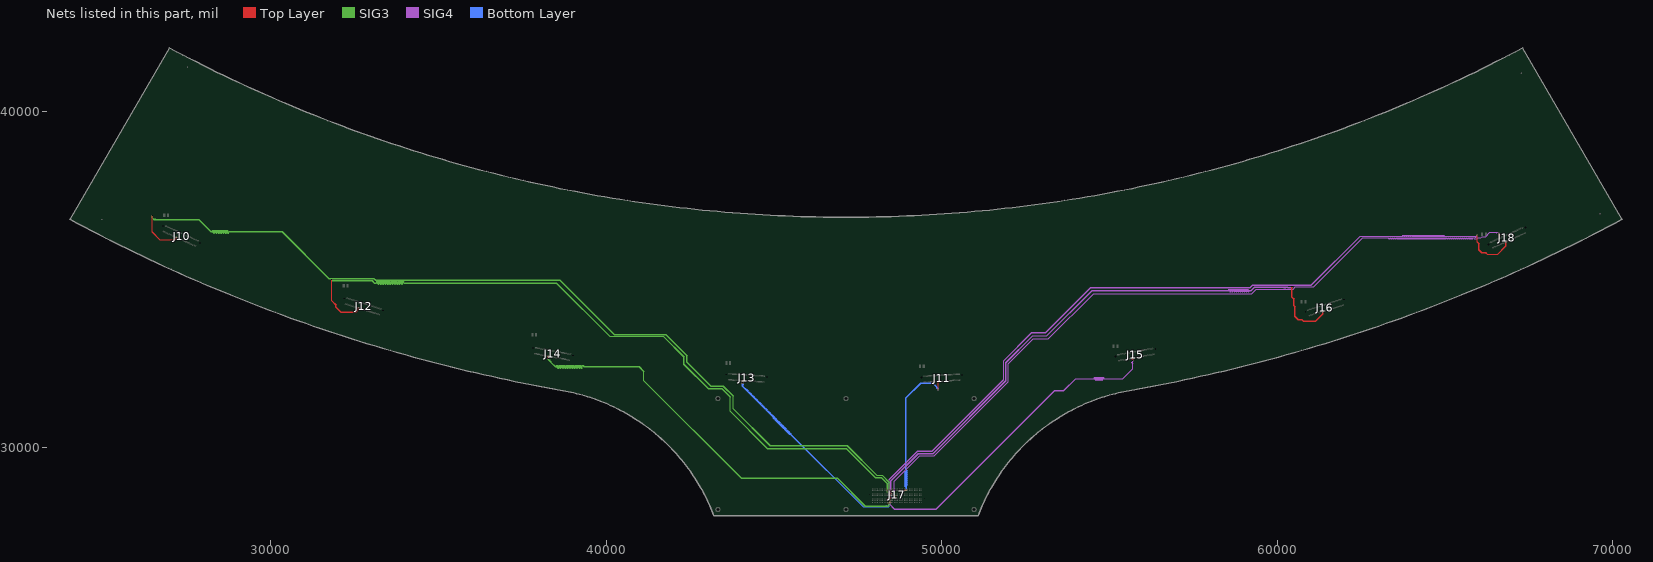
[diagram p0: the nets of this part, all layers, seen from the top]
# Altium PCB MISC86329.PcbDoc (part 7 of 11)
Units mil, origin at the board's own origin, x right, y up, seen from the top; angles counter-clockwise.
Board outline 46247.15 x 13937.21 mil, 6 copper layers (Top Layer, GND2, SIG3, SIG4, POWER5, Bottom Layer); 17 components, 210 nets, 908 pads, 1109 vias.

## Via types
v1: diameter 24, hole 12, Top Layer to Bottom Layer, 684 vias
v2: diameter 18, hole 9, Top Layer to Bottom Layer, 425 vias

## Nets (pads, with @x,y where several pads share a name; then routed paths per layer and width w, separated by ;. In a path a pad name is that pad's centre, name@x,y a point inside that pad or via, vN(x,y) a via of type N, cw(c..) or ccw(c..) an arc to the next point about the centre after c; other vN are vias at no path point) (continued)
DATAIN4P_CH7: J17.E16 J18.22 | length 23896.8
  Top Layer w5: v2(48614.09,28545) J17.E16@48637.89,28568.8 ; 66601,36381.5 66601,36360 66631.37,36329.63 J18.22@66631.37,36242.26
  SIG4 w5: v2(48614.09,28545) 48594.09,28565 48594.09,29002.09 49349,29757 49778.14,29757 51989,31967.86 51989,32495 52730,33236 53177.14,33236 54528.14,34587 59238.14,34587 59375.14,34724 60473.14,34724 60535.14,34786 61082.14,34786 62541.14,36245 63312.43,36245 63317,36240.43 63317,36225.43 63327.43,36215 63346.57,36215 63357,36225.43 63357,36240.43 63361.57,36245 63372.43,36245 63377,36240.43 63377,36225.43 63387.43,36215 63406.57,36215 63417,36225.43 63417,36240.43 63421.57,36245 63432.43,36245 63437,36240.43 63437,36225.43 63447.43,36215 63466.57,36215 63477,36225.43 63477,36240.43 63481.57,36245 63492.43,36245 63497,36240.43 63497,36225.43 63507.43,36215 63526.57,36215 63537,36225.43 63537,36240.43 63541.57,36245 63552.43,36245 63557,36240.43 63557,36225.43 63567.43,36215 63586.57,36215 63597,36225.43 63597,36240.43 63601.57,36245 63612.43,36245 63617,36240.43 63617,36225.43 63627.43,36215 63646.57,36215 63657,36225.43 63657,36240.43 63661.57,36245 63672.43,36245 63677,36240.43 63677,36225.43 63687.43,36215 63706.57,36215 63717,36225.43 63717,36240.43 63721.57,36245 63732.43,36245 63737,36240.43 63737,36225.43 63747.43,36215 63766.57,36215 63777,36225.43 63777,36240.43 63781.57,36245 63792.43,36245 63797,36240.43 63797,36225.43 63807.43,36215 63826.57,36215 63837,36225.43 63837,36240.43 63841.57,36245 63852.43,36245 63857,36240.43 63857,36225.43 63867.43,36215 63886.57,36215 63897,36225.43 63897,36240.43 63901.57,36245 63912.43,36245 63917,36240.43 63917,36225.43 63927.43,36215 63946.57,36215 63957,36225.43 63957,36240.43 63961.57,36245 63972.43,36245 63977,36240.43 63977,36225.43 63987.43,36215 64006.57,36215 64017,36225.43 64017,36240.43 64021.57,36245 64032.43,36245 64037,36240.43 64037,36225.43 64047.43,36215 64066.57,36215 64077,36225.43 64077,36240.43 64081.57,36245 64092.43,36245 64097,36240.43 64097,36225.43 64107.43,36215 64126.57,36215 64137,36225.43 64137,36240.43 64141.57,36245 64152.43,36245 64157,36240.43 64157,36225.43 64167.43,36215 64186.57,36215 64197,36225.43 64197,36240.43 64201.57,36245 64212.43,36245 64217,36240.43 64217,36225.43 64227.43,36215 64246.57,36215 64257,36225.43 64257,36240.43 64261.57,36245 64272.43,36245 64277,36240.43 64277,36225.43 64287.43,36215 64306.57,36215 64317,36225.43 64317,36240.43 64321.57,36245 64332.43,36245 64337,36240.43 64337,36225.43 64347.43,36215 64366.57,36215 64377,36225.43 64377,36240.43 64381.57,36245 64392.43,36245 64397,36240.43 64397,36225.43 64407.43,36215 64426.57,36215 64437,36225.43 64437,36240.43 64441.57,36245 64452.43,36245 64457,36240.43 64457,36225.43 64467.43,36215 64486.57,36215 64497,36225.43 64497,36240.43 64501.57,36245 64512.43,36245 64517,36240.43 64517,36225.43 64527.43,36215 64546.57,36215 64557,36225.43 64557,36240.43 64561.57,36245 64572.43,36245 64577,36240.43 64577,36225.43 64587.43,36215 64606.57,36215 64617,36225.43 64617,36240.43 64621.57,36245 64632.43,36245 64637,36240.43 64637,36225.43 64647.43,36215 64666.57,36215 64677,36225.43 64677,36240.43 64681.57,36245 64692.43,36245 64697,36240.43 64697,36225.43 64707.43,36215 64726.57,36215 64737,36225.43 64737,36240.43 64741.57,36245 64752.43,36245 64757,36240.43 64757,36225.43 64767.43,36215 64786.57,36215 64797,36225.43 64797,36240.43 64801.57,36245 64812.43,36245 64817,36240.43 64817,36225.43 64827.43,36215 64846.57,36215 64857,36225.43 64857,36240.43 64861.57,36245 64872.43,36245 64877,36240.43 64877,36225.43 64887.43,36215 64906.57,36215 64917,36225.43 64917,36240.43 64921.57,36245 64932.43,36245 64937,36240.43 64937,36225.43 64947.43,36215 64966.57,36215 64977,36225.43 64977,36240.43 64981.57,36245 64992.43,36245 64997,36240.43 64997,36225.43 65007.43,36215 65026.57,36215 65037,36225.43 65037,36240.43 65041.57,36245 65052.43,36245 65057,36240.43 65057,36225.43 65067.43,36215 65086.57,36215 65097,36225.43 65097,36240.43 65101.57,36245 65112.43,36245 65117,36240.43 65117,36225.43 65127.43,36215 65146.57,36215 65157,36225.43 65157,36240.43 65161.57,36245 65172.43,36245 65177,36240.43 65177,36225.43 65187.43,36215 65206.57,36215 65217,36225.43 65217,36240.43 65221.57,36245 65232.43,36245 65237,36240.43 65237,36225.43 65247.43,36215 65266.57,36215 65277,36225.43 65277,36240.43 65281.57,36245 65292.43,36245 65297,36240.43 65297,36225.43 65307.43,36215 65326.57,36215 65337,36225.43 65337,36240.43 65341.57,36245 65352.43,36245 65357,36240.43 65357,36225.43 65367.43,36215 65386.57,36215 65397,36225.43 65397,36240.43 65401.57,36245 65412.43,36245 65417,36240.43 65417,36225.43 65427.43,36215 65446.57,36215 65457,36225.43 65457,36240.43 65461.57,36245 65472.43,36245 65477,36240.43 65477,36225.43 65487.43,36215 65506.57,36215 65517,36225.43 65517,36240.43 65521.57,36245 65532.43,36245 65537,36240.43 65537,36225.43 65547.43,36215 65566.57,36215 65577,36225.43 65577,36240.43 65581.57,36245 65592.43,36245 65597,36240.43 65597,36225.43 65607.43,36215 65626.57,36215 65637,36225.43 65637,36240.43 65641.57,36245 65652.43,36245 65657,36240.43 65657,36225.43 65667.43,36215 65686.57,36215 65697,36225.43 65697,36240.43 65701.57,36245 65712.43,36245 65717,36240.43 65717,36225.43 65727.43,36215 65746.57,36215 65757,36225.43 65757,36240.43 65761.57,36245 65772.43,36245 65777,36240.43 65777,36225.43 65787.43,36215 65806.57,36215 65817,36225.43 65817,36240.43 65821.57,36245 65857.86,36245 65875.86,36227 65959.14,36227 65977.14,36245 66058.14,36245 66102.14,36289 66204.14,36289 66337.14,36422 66521,36422 66526,36417 66526,36402.15 66531,36397.15 66541,36397.15 66546,36402.15 66546,36417 66551,36422 66582.86,36422 66600,36404.86 66600,36396 v2@66595,36391
  other v2: 66594.5,36388
DATAIN5N_CH0: J10.29 J17.G20 | length 28227.2
  Top Layer w5: v2(26465.5,36917) 26472,36910.5 26472,36420.86 26703.86,36189 27155.14,36189 27186.72,36220.57 27186.72,36238.96 J10.29@27205.36,36257.61 ; v2(48414.09,28692.61) J17.G20@48437.89,28668.8
  SIG3 w5: v2(26465.5,36917) 26472,36910.5 26472,36846.86 26526.86,36792 26555,36792 27858.86,36792 28221.86,36429 28261.82,36429 28273.5,36440.68 28273.5,36461.49 28279.32,36467.31 28292.68,36467.31 28298.5,36461.49 28298.5,36402.37 28310.18,36390.69 28331.82,36390.69 28343.5,36402.37 28343.5,36461.49 28349.32,36467.31 28362.68,36467.31 28368.5,36461.49 28368.5,36402.37 28380.18,36390.69 28401.82,36390.69 28413.5,36402.37 28413.5,36461.49 28419.32,36467.31 28432.68,36467.31 28438.5,36461.49 28438.5,36402.37 28450.18,36390.69 28471.82,36390.69 28483.5,36402.37 28483.5,36461.49 28489.32,36467.31 28502.68,36467.31 28508.5,36461.49 28508.5,36402.37 28520.18,36390.69 28541.82,36390.69 28553.5,36402.37 28553.5,36461.49 28559.32,36467.31 28572.68,36467.31 28578.5,36461.49 28578.5,36402.37 28590.18,36390.69 28611.82,36390.69 28623.5,36402.37 28623.5,36461.49 28629.32,36467.31 28642.68,36467.31 28648.5,36461.49 28648.5,36402.37 28660.18,36390.69 28681.82,36390.69 28693.5,36402.37 28693.5,36461.49 28699.32,36467.31 28712.68,36467.31 28718.5,36461.49 28718.5,36402.37 28730.18,36390.69 28751.82,36390.69 28763.5,36402.37 28763.5,36423.18 28769.32,36429 30341.86,36429 31734.86,35036 33075.86,35036 33127.86,34984 38619.86,34984 40240.86,33363 41778,33363 42407,32734 42407,32544.86 43117.86,31834 43484,31834 43784,31534 43784,31158.86 44883.86,30059 47176,30059 48067,29168 48224.86,29168 48434.09,28958.77 48434.09,28712.61 v2(48414.09,28692.61)
DATAIN5N_CH1: J12.29 J17.F20 | length 23094.9
  Top Layer w5: v2(31815.5,35011) 31822,35004.5 31822,34375 31951,34246 31951,34175.86 32089.86,34037 32554.14,34037 32623.14,34106 32623.14,34130.56 J12.29@32643.17,34150.59 ; v2(48414.09,28642.61) J17.F20@48437.89,28618.8
  SIG3 w5: v2(31815.5,35011) 31822,35004.5 31822,34989.86 31838.86,34973 31862,34973 31867,34968 31888,34968 31893,34973 33022.86,34973 33093.86,34902 33158.82,34902 33170.5,34913.68 33170.5,34935.94 33176.32,34941.76 33189.68,34941.76 33195.5,34935.94 33195.5,34873.92 33207.18,34862.24 33228.82,34862.24 33240.5,34873.92 33240.5,34935.94 33246.32,34941.76 33259.68,34941.76 33265.5,34935.94 33265.5,34873.92 33277.18,34862.24 33298.82,34862.24 33310.5,34873.92 33310.5,34935.94 33316.32,34941.76 33329.68,34941.76 33335.5,34935.94 33335.5,34873.92 33347.18,34862.24 33368.82,34862.24 33380.5,34873.92 33380.5,34935.94 33386.32,34941.76 33399.68,34941.76 33405.5,34935.94 33405.5,34873.92 33417.18,34862.24 33438.82,34862.24 33450.5,34873.92 33450.5,34935.94 33456.32,34941.76 33469.68,34941.76 33475.5,34935.94 33475.5,34873.92 33487.18,34862.24 33508.82,34862.24 33520.5,34873.92 33520.5,34935.94 33526.32,34941.76 33539.68,34941.76 33545.5,34935.94 33545.5,34873.92 33557.18,34862.24 33578.82,34862.24 33590.5,34873.92 33590.5,34935.94 33596.32,34941.76 33609.68,34941.76 33615.5,34935.94 33615.5,34873.92 33627.18,34862.24 33648.82,34862.24 33660.5,34873.92 33660.5,34935.94 33666.32,34941.76 33679.68,34941.76 33685.5,34935.94 33685.5,34873.92 33697.18,34862.24 33718.82,34862.24 33730.5,34873.92 33730.5,34935.94 33736.32,34941.76 33749.68,34941.76 33755.5,34935.94 33755.5,34873.92 33767.18,34862.24 33788.82,34862.24 33800.5,34873.92 33800.5,34935.94 33806.32,34941.76 33819.68,34941.76 33825.5,34935.94 33825.5,34873.92 33837.18,34862.24 33858.82,34862.24 33870.5,34873.92 33870.5,34935.94 33876.32,34941.76 33889.68,34941.76 33895.5,34935.94 33895.5,34873.92 33907.18,34862.24 33928.82,34862.24 33940.5,34873.92 33940.5,34935.94 33946.32,34941.76 33959.68,34941.76 33965.5,34935.94 33965.5,34913.68 33977.18,34902 38516.86,34902 40108.86,33310 41706,33310 42318,32698 42318,32472.86 43038.86,31752 43447,31752 43694,31505 43694,31074.86 44802.86,29966 47153.86,29966 48014.86,29105 48195.86,29105 48385,28915.86 48385,28674 48406.96,28652.04 48414.09,28644.91 v2(48414.09,28642.61)
DATAIN5N_CH2: J14.29 J17.B20 | length 13805.4
  Top Layer w5: v2(38289.5,32657) 38283,32663.5 38283,32689 38293,32699 J14.29@38293,32716 ; v2(48414.09,28395) J17.B20@48437.89,28418.8
  SIG3 w5: v2@38287,32654 38282,32649 38282,32624 38296.42,32609.58 38305.26,32609.58 38308.78,32613.1 38317.62,32613.1 38326.46,32604.26 38326.46,32595.42 38322.94,32591.9 38322.94,32583.06 38331.77,32574.23 38340.61,32574.23 38344.13,32577.75 38352.97,32577.75 38361.81,32568.91 38361.81,32560.07 38358.29,32556.55 38358.29,32547.71 38490,32416 38511.68,32416 38517.5,32421.82 38517.5,32436.85 38529.18,32448.52 38550.82,32448.52 38562.5,32436.85 38562.5,32382.3 38568.32,32376.48 38581.68,32376.48 38587.5,32382.3 38587.5,32436.85 38599.18,32448.52 38620.82,32448.52 38632.5,32436.85 38632.5,32382.3 38638.32,32376.48 38651.68,32376.48 38657.5,32382.3 38657.5,32436.85 38669.18,32448.52 38690.82,32448.52 38702.5,32436.85 38702.5,32382.3 38708.32,32376.48 38721.68,32376.48 38727.5,32382.3 38727.5,32436.85 38739.18,32448.52 38760.82,32448.52 38772.5,32436.85 38772.5,32382.3 38778.32,32376.48 38791.68,32376.48 38797.5,32382.3 38797.5,32436.85 38809.18,32448.52 38830.82,32448.52 38842.5,32436.85 38842.5,32382.3 38848.32,32376.48 38861.68,32376.48 38867.5,32382.3 38867.5,32436.85 38879.18,32448.52 38900.82,32448.52 38912.5,32436.85 38912.5,32382.3 38918.32,32376.48 38931.68,32376.48 38937.5,32382.3 38937.5,32436.85 38949.18,32448.52 38970.82,32448.52 38982.5,32436.85 38982.5,32382.3 38988.32,32376.48 39001.68,32376.48 39007.5,32382.3 39007.5,32436.85 39019.18,32448.52 39040.82,32448.52 39052.5,32436.85 39052.5,32382.3 39058.32,32376.48 39071.68,32376.48 39077.5,32382.3 39077.5,32436.85 39089.18,32448.52 39110.82,32448.52 39122.5,32436.85 39122.5,32382.3 39128.32,32376.48 39141.68,32376.48 39147.5,32382.3 39147.5,32436.85 39159.18,32448.52 39180.82,32448.52 39192.5,32436.85 39192.5,32382.3 39198.32,32376.48 39211.68,32376.48 39217.5,32382.3 39217.5,32436.85 39229.18,32448.52 39250.82,32448.52 39262.5,32436.85 39262.5,32382.3 39268.32,32376.48 39281.68,32376.48 39287.5,32382.3 39287.5,32436.85 39299.18,32448.52 39320.82,32448.52 39332.5,32436.85 39332.5,32421.82 39338.32,32416 40982.14,32416 41129,32269.14 41129,31998 44032,29095 46891,29095 47717,28269 48400,28269 48434.09,28303.09 48434.09,28375 v2(48414.09,28395)
DATAIN5N_CH3: J13.29 J17.A20 | length 7749.4
  Top Layer w5: 44072.53,31936.5 44072.53,31954.28 44083.25,31965 J13.29@44083.25,31993.07 ; v2(48414.09,28345) J17.A20@48437.89,28368.8
  Bottom Layer w5: v2@44078,31927 44076,31927 44072.53,31923.53 44072.53,31923.17 44072,31922.63 44072,31897.5 44077,31892.5 44090.54,31892.5 44095.54,31887.5 44095.54,31872.5 44090.54,31867.5 44077,31867.5 44072,31862.5 44072,31828.14 44131.03,31769.12 44135.72,31769.12 44141.03,31774.42 44154.01,31774.42 44165.77,31762.65 44165.77,31749.67 44160.47,31744.37 44160.47,31739.67 44166.38,31733.76 44171.08,31733.76 44176.38,31739.06 44189.36,31739.06 44201.13,31727.3 44201.13,31714.32 44195.83,31709.01 44195.83,31704.32 44201.74,31698.41 44206.43,31698.41 44211.74,31703.71 44224.72,31703.71 44236.49,31691.94 44236.49,31678.96 44231.18,31673.66 44231.18,31668.96 44237.09,31663.05 44241.79,31663.05 44247.09,31668.35 44260.07,31668.35 44271.84,31656.59 44271.84,31643.6 44266.54,31638.3 44266.54,31633.6 44272.45,31627.69 44277.14,31627.69 44282.45,31633 44295.43,31633 44307.2,31621.23 44307.2,31608.25 44301.89,31602.95 44301.89,31598.25 44307.8,31592.34 44312.5,31592.34 44317.8,31597.64 44330.78,31597.64 44342.55,31585.88 44342.55,31572.89 44337.25,31567.59 44337.25,31562.89 44343.16,31556.98 44347.85,31556.98 44353.16,31562.29 44366.14,31562.29 44377.91,31550.52 44377.91,31537.54 44372.6,31532.24 44372.6,31527.54 44378.51,31521.63 44383.21,31521.63 44388.51,31526.93 44401.49,31526.93 44413.26,31515.16 44413.26,31502.18 44407.96,31496.88 44407.96,31492.18 44413.87,31486.27 44418.57,31486.27 44423.87,31491.58 44436.85,31491.58 44448.62,31479.81 44448.62,31466.83 44443.31,31461.52 44443.31,31456.83 44449.22,31450.92 44453.92,31450.92 44459.22,31456.22 44472.2,31456.22 44483.97,31444.45 44483.97,31431.47 44478.67,31426.17 44478.67,31421.47 44484.58,31415.56 44489.28,31415.56 44494.58,31420.87 44507.56,31420.87 44519.33,31409.1 44519.33,31396.12 44514.02,31390.81 44514.02,31386.12 44519.93,31380.21 44524.63,31380.21 44529.93,31385.51 44542.92,31385.51 44554.68,31373.74 44554.68,31360.76 44549.38,31355.46 44549.38,31350.76 44555.29,31344.85 44559.99,31344.85 44565.29,31350.16 44578.27,31350.16 44590.04,31338.39 44590.04,31325.41 44584.74,31320.1 44584.74,31315.41 44590.65,31309.5 44595.34,31309.5 44600.65,31314.8 44613.63,31314.8 44625.39,31303.03 44625.39,31290.05 44620.09,31284.75 44620.09,31280.05 44626,31274.14 44630.7,31274.14 44636,31279.44 44648.98,31279.44 44660.75,31267.68 44660.75,31254.7 44655.45,31249.39 44655.45,31244.7 44661.36,31238.79 44666.05,31238.79 44671.36,31244.09 44684.34,31244.09 44696.1,31232.32 44696.1,31219.34 44690.8,31214.04 44690.8,31209.34 44696.71,31203.43 44701.41,31203.43 44706.71,31208.73 44719.69,31208.73 44731.46,31196.97 44731.46,31183.99 44726.16,31178.68 44726.16,31173.99 44732.07,31168.08 44736.76,31168.08 44742.07,31173.38 44755.05,31173.38 44766.82,31161.61 44766.82,31148.63 44761.51,31143.33 44761.51,31138.63 44767.42,31132.72 44772.12,31132.72 44777.42,31138.02 44790.4,31138.02 44802.17,31126.26 44802.17,31113.27 44796.87,31107.97 44796.87,31103.27 44802.78,31097.36 44807.47,31097.36 44812.78,31102.67 44825.76,31102.67 44837.53,31090.9 44837.53,31077.92 44832.22,31072.62 44832.22,31067.92 44838.13,31062.01 44842.83,31062.01 44848.13,31067.31 44861.11,31067.31 44872.88,31055.54 44872.88,31042.56 44867.58,31037.26 44867.58,31032.56 44873.49,31026.65 44878.18,31026.65 44883.49,31031.96 44896.47,31031.96 44908.24,31020.19 44908.24,31007.21 44902.93,31001.91 44902.93,30997.21 44908.84,30991.3 44913.54,30991.3 44918.84,30996.6 44931.82,30996.6 44943.59,30984.83 44943.59,30971.85 44938.29,30966.55 44938.29,30961.85 44944.2,30955.94 44948.9,30955.94 44954.2,30961.25 44967.18,30961.25 44978.95,30949.48 44978.95,30936.5 44973.64,30931.19 44973.64,30926.5 44979.55,30920.59 44984.25,30920.59 44989.55,30925.89 45002.54,30925.89 45014.3,30914.12 45014.3,30901.14 44994.86,30881.7 44994.86,30877 45000.77,30871.09 45005.46,30871.09 45024.91,30890.54 45037.89,30890.54 45049.66,30878.77 45049.66,30865.79 45030.21,30846.34 45030.21,30841.65 45036.12,30835.74 45040.82,30835.74 45060.26,30855.18 45073.25,30855.18 45085.01,30843.41 45085.01,30830.43 45065.57,30810.99 45065.57,30806.29 45071.48,30800.38 45076.17,30800.38 45095.62,30819.83 45108.6,30819.83 45120.37,30808.06 45120.37,30795.08 45100.92,30775.63 45100.92,30770.93 45106.83,30765.02 45111.53,30765.02 45130.98,30784.47 45143.96,30784.47 45155.72,30772.7 45155.72,30759.72 45136.28,30740.28 45136.28,30735.58 45142.19,30729.67 45146.89,30729.67 45166.33,30749.11 45179.31,30749.11 45191.08,30737.35 45191.08,30724.37 45171.63,30704.92 45171.63,30700.22 45177.54,30694.31 45182.24,30694.31 45201.69,30713.76 45214.67,30713.76 45226.43,30701.99 45226.43,30689.01 45206.99,30669.56 45206.99,30664.87 45212.9,30658.96 45217.6,30658.96 45237.04,30678.4 45250.02,30678.4 45261.79,30666.64 45261.79,30653.66 45242.34,30634.21 45242.34,30629.51 45248.25,30623.6 45252.95,30623.6 45272.4,30643.05 45285.38,30643.05 45297.15,30631.28 45297.15,30618.3 45277.7,30598.85 45277.7,30594.16 45283.61,30588.25 45288.31,30588.25 45307.75,30607.69 45320.73,30607.69 45332.5,30595.93 45332.5,30582.94 45313.06,30563.5 45313.06,30558.8 45318.97,30552.89 45323.66,30552.89 45343.11,30572.34 45356.09,30572.34 45367.86,30560.57 45367.86,30547.59 45348.41,30528.14 45348.41,30523.45 45354.32,30517.54 45359.02,30517.54 45378.46,30536.98 45391.44,30536.98 45403.21,30525.21 45403.21,30512.23 45383.77,30492.79 45383.77,30488.09 45389.68,30482.18 45394.37,30482.18 45413.82,30501.63 45426.8,30501.63 45438.57,30489.86 45438.57,30476.88 45419.12,30457.43 45419.12,30452.74 45425.03,30446.83 45429.73,30446.83 45449.17,30466.27 45462.15,30466.27 45473.92,30454.5 45473.92,30441.52 45454.48,30422.08 45454.48,30417.38 45460.39,30411.47 45465.08,30411.47 45481.61,30428 45500.43,30428 45510,30418.43 45510,30390.14 47660.14,28240 48331.18,28240 48334.5,28243.32 48334.5,28250.82 48343.68,28260 48360.32,28260 48369.5,28250.82 48369.5,28243.32 48372.82,28240 48412,28240 48435,28263 48435,28324.09 v2(48414.09,28345)
  other v2: 44079.03,31930
DATAIN5N_CH4: J11.29 J17.H11 | length 5093.6
  Top Layer w5: J17.H11@48887.89,28718.8 v2(48911.69,28742.61) ; 49904.25,31721.5 49904.25,31939.28 49914.97,31950 J11.29@49914.97,31974.73
  Bottom Layer w5: v2(48911.69,28742.61) 48931.69,28762.61 48931.69,28828.93 48925.62,28835 48913.62,28835 48901.69,28846.93 48901.69,28863.07 48913.62,28875 48955.62,28875 48961.69,28881.07 48961.69,28888.93 48955.62,28895 48913.62,28895 48901.69,28906.93 48901.69,28923.07 48913.62,28935 48955.62,28935 48961.69,28941.07 48961.69,28948.93 48955.62,28955 48913.62,28955 48901.69,28966.93 48901.69,28983.07 48913.62,28995 48955.62,28995 48961.69,29001.07 48961.69,29008.93 48955.62,29015 48913.62,29015 48901.69,29026.93 48901.69,29043.07 48913.62,29055 48955.62,29055 48961.69,29061.07 48961.69,29068.93 48955.62,29075 48913.62,29075 48901.69,29086.93 48901.69,29103.07 48913.62,29115 48955.62,29115 48961.69,29121.07 48961.69,29128.93 48955.62,29135 48913.62,29135 48901.69,29146.93 48901.69,29163.07 48913.62,29175 48955.62,29175 48961.69,29181.07 48961.69,29188.93 48955.62,29195 48913.62,29195 48901.69,29206.93 48901.69,29223.07 48913.62,29235 48955.62,29235 48961.69,29241.07 48961.69,29248.93 48955.62,29255 48913.62,29255 48901.69,29266.93 48901.69,29283.07 48913.62,29295 48955.62,29295 48961.69,29301.07 48961.69,29308.93 48955.62,29315 48949,29315 48931.69,29332.31 48931.69,31481.69 49381,31931 49738.14,31931 49904,31765.14 49904,31722.09 49904.25,31721.83 49904.25,31721.75 v2@49909,31717
  other v2: 49910.75,31715
DATAIN5N_CH5: J15.29 J17.C20 | length 10126.3
  Top Layer w5: v2(48414.09,28445) J17.C20@48437.89,28468.8 ; 55697,32596.5 55697,32632.54 55705.46,32641 J15.29@55705.46,32667.24
  SIG4 w5: v2(48414.09,28445) 48434.09,28425 48434.09,28319.77 48589.86,28164 49842.14,28164 53370.14,31692 53639.14,31692 53993.14,32046 54544.57,32046 54555,32056.43 54555,32079.24 54559.57,32083.81 54570.43,32083.81 54575,32079.24 54575,32020.62 54585.43,32010.19 54604.57,32010.19 54615,32020.62 54615,32079.24 54619.57,32083.81 54630.43,32083.81 54635,32079.24 54635,32020.62 54645.43,32010.19 54664.57,32010.19 54675,32020.62 54675,32079.24 54679.57,32083.81 54690.43,32083.81 54695,32079.24 54695,32020.62 54705.43,32010.19 54724.57,32010.19 54735,32020.62 54735,32079.24 54739.57,32083.81 54750.43,32083.81 54755,32079.24 54755,32020.62 54765.43,32010.19 54784.57,32010.19 54795,32020.62 54795,32079.24 54799.57,32083.81 54810.43,32083.81 54815,32079.24 54815,32056.43 54825.43,32046 55400.14,32046 55696,32341.86 55696,32463 55696,32517 55696,32547 55696,32562 55696,32572 55696,32582.17 55703.5,32589.67 v2(55703.5,32590)
DATAIN5N_CH6: J16.29 J17.D20 | length 18292.6
  Top Layer w5: v2(48414.09,28495) J17.D20@48437.89,28518.8 ; 60436,34792.5 60436,34479.86 60491,34424.86 60491,34219 60525,34185 60525,33904.86 60614.86,33815 60723.86,33815 60773.86,33765 61148.14,33765 61367,33983.86 61367,34032.61 ; 61368.39,34034 J16.29@61368.39,34060.27
  SIG4 w5: v2(48414.09,28495) 48440.75,28495 48457.25,28511.5 48466.44,28511.5 48484,28529.06 48484,29009.14 49306.86,29832 49742,29832 51910,32000 51910,32535 52712,33337 53130,33337 54483,34690 58545.43,34690 58550,34694.57 58550,34709.57 58560.43,34720 58579.57,34720 58590,34709.57 58590,34664.57 58594.57,34660 58605.43,34660 58610,34664.57 58610,34709.57 58620.43,34720 58639.57,34720 58650,34709.57 58650,34664.57 58654.57,34660 58665.43,34660 58670,34664.57 58670,34709.57 58680.43,34720 58699.57,34720 58710,34709.57 58710,34664.57 58714.57,34660 58725.43,34660 58730,34664.57 58730,34709.57 58740.43,34720 58759.57,34720 58770,34709.57 58770,34664.57 58774.57,34660 58785.43,34660 58790,34664.57 58790,34709.57 58800.43,34720 58819.57,34720 58830,34709.57 58830,34664.57 58834.57,34660 58845.43,34660 58850,34664.57 58850,34709.57 58860.43,34720 58879.57,34720 58890,34709.57 58890,34664.57 58894.57,34660 58905.43,34660 58910,34664.57 58910,34709.57 58920.43,34720 58939.57,34720 58950,34709.57 58950,34664.57 58954.57,34660 58965.43,34660 58970,34664.57 58970,34709.57 58980.43,34720 58999.57,34720 59010,34709.57 59010,34664.57 59014.57,34660 59025.43,34660 59030,34664.57 59030,34709.57 59040.43,34720 59059.57,34720 59070,34709.57 59070,34664.57 59074.57,34660 59085.43,34660 59090,34664.57 59090,34709.57 59100.43,34720 59119.57,34720 59130,34709.57 59130,34664.57 59134.57,34660 59145.43,34660 59150,34664.57 59150,34679.57 59160.43,34690 59222,34690 59325,34793 60078,34793 60192,34793 60222,34793 60232,34793 60291.14,34793 60313.14,34771 60422.86,34771 60436,34784.14 60436,34792 v2@60432,34796
  other v2: 60429.5,34799
DATAIN5N_CH7: J17.E20 J18.29 | length 23890.7
  Top Layer w5: v2(48414.09,28545) J17.E20@48437.89,28568.8 ; v2(65945.5,36331) 65952,36324.5 65952,36125 66010,36067 66010,35882.86 66080.86,35812 66202.86,35812 66258.86,35756 66573.14,35756 66824,36006.86 66824,36100.84 66819.09,36105.75 66819.34,36106 J18.29@66819.34,36133.06
  SIG4 w5: v2(48414.09,28545) 48434.09,28565 48434.09,29051.23 49289.86,29907 49721,29907 51843,32029 51843,32594 52685,33436 53098,33436 54436,34774 59190,34774 59264,34848 61015,34848 62467,36300 63730.93,36300 63734,36303.07 63734,36319.57 63744.43,36330 63763.57,36330 63774,36319.57 63774,36304.57 63778.57,36300 63789.43,36300 63794,36304.57 63794,36319.57 63804.43,36330 63823.57,36330 63834,36319.57 63834,36304.57 63838.57,36300 63849.43,36300 63854,36304.57 63854,36319.57 63864.43,36330 63883.57,36330 63894,36319.57 63894,36304.57 63898.57,36300 63909.43,36300 63914,36304.57 63914,36319.57 63924.43,36330 63943.57,36330 63954,36319.57 63954,36304.57 63958.57,36300 63969.43,36300 63974,36304.57 63974,36319.57 63984.43,36330 64003.57,36330 64014,36319.57 64014,36304.57 64018.57,36300 64029.43,36300 64034,36304.57 64034,36319.57 64044.43,36330 64063.57,36330 64074,36319.57 64074,36304.57 64078.57,36300 64089.43,36300 64094,36304.57 64094,36319.57 64104.43,36330 64123.57,36330 64134,36319.57 64134,36304.57 64138.57,36300 64149.43,36300 64154,36304.57 64154,36319.57 64164.43,36330 64183.57,36330 64194,36319.57 64194,36304.57 64198.57,36300 64209.43,36300 64214,36304.57 64214,36319.57 64224.43,36330 64243.57,36330 64254,36319.57 64254,36304.57 64258.57,36300 64269.43,36300 64274,36304.57 64274,36319.57 64284.43,36330 64303.57,36330 64314,36319.57 64314,36304.57 64318.57,36300 64329.43,36300 64334,36304.57 64334,36319.57 64344.43,36330 64363.57,36330 64374,36319.57 64374,36304.57 64378.57,36300 64389.43,36300 64394,36304.57 64394,36319.57 64404.43,36330 64423.57,36330 64434,36319.57 64434,36304.57 64438.57,36300 64449.43,36300 64454,36304.57 64454,36319.57 64464.43,36330 64483.57,36330 64494,36319.57 64494,36304.57 64498.57,36300 64509.43,36300 64514,36304.57 64514,36319.57 64524.43,36330 64543.57,36330 64554,36319.57 64554,36304.57 64558.57,36300 64569.43,36300 64574,36304.57 64574,36319.57 64584.43,36330 64603.57,36330 64614,36319.57 64614,36304.57 64618.57,36300 64629.43,36300 64634,36304.57 64634,36319.57 64644.43,36330 64663.57,36330 64674,36319.57 64674,36304.57 64678.57,36300 64689.43,36300 64694,36304.57 64694,36319.57 64704.43,36330 64723.57,36330 64734,36319.57 64734,36304.57 64738.57,36300 64749.43,36300 64754,36304.57 64754,36319.57 64764.43,36330 64783.57,36330 64794,36319.57 64794,36304.57 64798.57,36300 64809.43,36300 64814,36304.57 64814,36319.57 64824.43,36330 64843.57,36330 64854,36319.57 64854,36304.57 64858.57,36300 64869.43,36300 64874,36304.57 64874,36319.57 64884.43,36330 64903.57,36330 64914,36319.57 64914,36304.57 64918.57,36300 64929.43,36300 64934,36304.57 64934,36319.57 64944.43,36330 64963.57,36330 64974,36319.57 64974,36304.57 64978.57,36300 65800,36300 65896,36300 65942,36300 65952,36310 65952,36323 v2@65946,36329
DATAIN5P_CH0: J10.27 J17.G19 | length 28226.8
  Top Layer w5: v2(26488.5,36917) 26482,36910.5 26482,36425 26708,36199 27151,36199 27176.72,36224.72 J10.27@27176.72,36270.7 ; v2(48464.09,28692.61) J17.G19@48487.89,28668.8
  SIG3 w5: v2(26488.5,36917) 26482,36910.5 26482,36851 26531,36802 26555,36802 26560,36807 26560,36816.56 26565,36821.56 26575,36821.56 26580,36816.56 26580,36807 26585,36802 27863,36802 28226,36439 28257.68,36439 28263.5,36444.82 28263.5,36465.63 28275.18,36477.31 28296.82,36477.31 28308.5,36465.63 28308.5,36406.51 28314.32,36400.69 28327.68,36400.69 28333.5,36406.51 28333.5,36465.63 28345.18,36477.31 28366.82,36477.31 28378.5,36465.63 28378.5,36406.51 28384.32,36400.69 28397.68,36400.69 28403.5,36406.51 28403.5,36465.63 28415.18,36477.31 28436.82,36477.31 28448.5,36465.63 28448.5,36406.51 28454.32,36400.69 28467.68,36400.69 28473.5,36406.51 28473.5,36465.63 28485.18,36477.31 28506.82,36477.31 28518.5,36465.63 28518.5,36406.51 28524.32,36400.69 28537.68,36400.69 28543.5,36406.51 28543.5,36465.63 28555.18,36477.31 28576.82,36477.31 28588.5,36465.63 28588.5,36406.51 28594.32,36400.69 28607.68,36400.69 28613.5,36406.51 28613.5,36465.63 28625.18,36477.31 28646.82,36477.31 28658.5,36465.63 28658.5,36406.51 28664.32,36400.69 28677.68,36400.69 28683.5,36406.51 28683.5,36465.63 28695.18,36477.31 28716.82,36477.31 28728.5,36465.63 28728.5,36406.51 28734.32,36400.69 28747.68,36400.69 28753.5,36406.51 28753.5,36427.32 28765.18,36439 30346,36439 31739,35046 33080,35046 33132,34994 38624,34994 40245,33373 41782.14,33373 42417,32738.14 42417,32549 43122,31844 43488.14,31844 43794,31538.14 43794,31163 44888,30069 47180.14,30069 48071.14,29178 48229,29178 48444.09,28962.91 48444.09,28712.61 v2(48464.09,28692.61)
DATAIN5P_CH1: J12.27 J17.F19 | length 23095.1
  Top Layer w5: v2(31838.5,35011) 31832,35004.5 31832,34379.14 31961,34250.14 31961,34180 32094,34047 32550,34047 32613.14,34110.14 J12.27@32613.14,34160.1 ; v2(48464.09,28642.61) J17.F19@48487.89,28618.8
  SIG3 w5: v2(31838.5,35011) 31832,35004.5 31832,34994 31843,34983 31862,34983 33027,34983 33098,34912 33154.68,34912 33160.5,34917.82 33160.5,34940.08 33172.18,34951.76 33193.82,34951.76 33205.5,34940.08 33205.5,34878.06 33211.32,34872.24 33224.68,34872.24 33230.5,34878.06 33230.5,34940.08 33242.18,34951.76 33263.82,34951.76 33275.5,34940.08 33275.5,34878.06 33281.32,34872.24 33294.68,34872.24 33300.5,34878.06 33300.5,34940.08 33312.18,34951.76 33333.82,34951.76 33345.5,34940.08 33345.5,34878.06 33351.32,34872.24 33364.68,34872.24 33370.5,34878.06 33370.5,34940.08 33382.18,34951.76 33403.82,34951.76 33415.5,34940.08 33415.5,34878.06 33421.32,34872.24 33434.68,34872.24 33440.5,34878.06 33440.5,34940.08 33452.18,34951.76 33473.82,34951.76 33485.5,34940.08 33485.5,34878.06 33491.32,34872.24 33504.68,34872.24 33510.5,34878.06 33510.5,34940.08 33522.18,34951.76 33543.82,34951.76 33555.5,34940.08 33555.5,34878.06 33561.32,34872.24 33574.68,34872.24 33580.5,34878.06 33580.5,34940.08 33592.18,34951.76 33613.82,34951.76 33625.5,34940.08 33625.5,34878.06 33631.32,34872.24 33644.68,34872.24 33650.5,34878.06 33650.5,34940.08 33662.18,34951.76 33683.82,34951.76 33695.5,34940.08 33695.5,34878.06 33701.32,34872.24 33714.68,34872.24 33720.5,34878.06 33720.5,34940.08 33732.18,34951.76 33753.82,34951.76 33765.5,34940.08 33765.5,34878.06 33771.32,34872.24 33784.68,34872.24 33790.5,34878.06 33790.5,34940.08 33802.18,34951.76 33823.82,34951.76 33835.5,34940.08 33835.5,34878.06 33841.32,34872.24 33854.68,34872.24 33860.5,34878.06 33860.5,34940.08 33872.18,34951.76 33893.82,34951.76 33905.5,34940.08 33905.5,34878.06 33911.32,34872.24 33924.68,34872.24 33930.5,34878.06 33930.5,34940.08 33942.18,34951.76 33963.82,34951.76 33975.5,34940.08 33975.5,34917.82 33981.32,34912 38521,34912 40113,33320 41710.14,33320 42328,32702.14 42328,32477 43043,31762 43451.14,31762 43704,31509.14 43704,31079 44807,29976 47158,29976 48019,29115 48200,29115 48395,28920 48395,28678.14 48414.04,28659.11 48420.92,28659.11 48437.42,28642.61 v2(48464.09,28642.61)
DATAIN5P_CH2: J14.27 J17.B19 | length 13806.6
  Top Layer w5: J14.27@38266.27,32727.75 38266.27,32702 38273,32695.27 38273,32663.5 ; v2(48464.09,28395) J17.B19@48487.89,28418.8
  SIG3 w5: v2(38266.5,32657) v2@38273,32657 ; v2@38267,32655 38272,32650 38272,32619.86 38485.86,32406 38515.82,32406 38527.5,32417.68 38527.5,32432.7 38533.32,32438.52 38546.68,32438.52 38552.5,32432.7 38552.5,32378.16 38564.18,32366.48 38585.82,32366.48 38597.5,32378.16 38597.5,32432.7 38603.32,32438.52 38616.68,32438.52 38622.5,32432.7 38622.5,32378.16 38634.18,32366.48 38655.82,32366.48 38667.5,32378.16 38667.5,32432.7 38673.32,32438.52 38686.68,32438.52 38692.5,32432.7 38692.5,32378.16 38704.18,32366.48 38725.82,32366.48 38737.5,32378.16 38737.5,32432.7 38743.32,32438.52 38756.68,32438.52 38762.5,32432.7 38762.5,32378.16 38774.18,32366.48 38795.82,32366.48 38807.5,32378.16 38807.5,32432.7 38813.32,32438.52 38826.68,32438.52 38832.5,32432.7 38832.5,32378.16 38844.18,32366.48 38865.82,32366.48 38877.5,32378.16 38877.5,32432.7 38883.32,32438.52 38896.68,32438.52 38902.5,32432.7 38902.5,32378.16 38914.18,32366.48 38935.82,32366.48 38947.5,32378.16 38947.5,32432.7 38953.32,32438.52 38966.68,32438.52 38972.5,32432.7 38972.5,32378.16 38984.18,32366.48 39005.82,32366.48 39017.5,32378.16 39017.5,32432.7 39023.32,32438.52 39036.68,32438.52 39042.5,32432.7 39042.5,32378.16 39054.18,32366.48 39075.82,32366.48 39087.5,32378.16 39087.5,32432.7 39093.32,32438.52 39106.68,32438.52 39112.5,32432.7 39112.5,32378.16 39124.18,32366.48 39145.82,32366.48 39157.5,32378.16 39157.5,32432.7 39163.32,32438.52 39176.68,32438.52 39182.5,32432.7 39182.5,32378.16 39194.18,32366.48 39215.82,32366.48 39227.5,32378.16 39227.5,32432.7 39233.32,32438.52 39246.68,32438.52 39252.5,32432.7 39252.5,32378.16 39264.18,32366.48 39285.82,32366.48 39297.5,32378.16 39297.5,32432.7 39303.32,32438.52 39316.68,32438.52 39322.5,32432.7 39322.5,32417.68 39334.18,32406 40978,32406 41119,32265 41119,31993.86 44027.86,29085 46886.86,29085 47712.86,28259 48404.14,28259 48444.09,28298.94 48444.09,28375 v2(48464.09,28395)
DATAIN5P_CH3: J13.27 J17.A19 | length 7749.8
  Top Layer w5: J13.27@44051.81,31995.03 44051.81,31970 44062.53,31959.28 44062.53,31936.5 ; v2(48464.09,28345) J17.A19@48487.89,28368.8
  Bottom Layer w5: v2@44057,31930 44062,31925 44062,31824 44126.88,31759.12 44139.86,31759.12 44145.17,31764.42 44149.86,31764.42 44155.77,31758.51 44155.77,31753.81 44150.47,31748.51 44150.47,31735.53 44162.24,31723.76 44175.22,31723.76 44180.52,31729.06 44185.22,31729.06 44191.13,31723.15 44191.13,31718.46 44185.83,31713.15 44185.83,31700.17 44197.59,31688.41 44210.58,31688.41 44215.88,31693.71 44220.58,31693.71 44226.49,31687.8 44226.49,31683.1 44221.18,31677.8 44221.18,31664.82 44232.95,31653.05 44245.93,31653.05 44251.23,31658.35 44255.93,31658.35 44261.84,31652.44 44261.84,31647.75 44256.54,31642.44 44256.54,31629.46 44268.31,31617.69 44281.29,31617.69 44286.59,31623 44291.29,31623 44297.2,31617.09 44297.2,31612.39 44291.89,31607.09 44291.89,31594.11 44303.66,31582.34 44316.64,31582.34 44321.94,31587.64 44326.64,31587.64 44332.55,31581.73 44332.55,31577.04 44327.25,31571.73 44327.25,31558.75 44339.02,31546.98 44352,31546.98 44357.3,31552.29 44362,31552.29 44367.91,31546.38 44367.91,31541.68 44362.6,31536.38 44362.6,31523.4 44374.37,31511.63 44387.35,31511.63 44392.66,31516.93 44397.35,31516.93 44403.26,31511.02 44403.26,31506.33 44397.96,31501.02 44397.96,31488.04 44409.73,31476.27 44422.71,31476.27 44428.01,31481.58 44432.71,31481.58 44438.62,31475.67 44438.62,31470.97 44433.31,31465.67 44433.31,31452.69 44445.08,31440.92 44458.06,31440.92 44463.37,31446.22 44468.06,31446.22 44473.97,31440.31 44473.97,31435.61 44468.67,31430.31 44468.67,31417.33 44480.44,31405.56 44493.42,31405.56 44498.72,31410.87 44503.42,31410.87 44509.33,31404.96 44509.33,31400.26 44504.02,31394.96 44504.02,31381.98 44515.79,31370.21 44528.77,31370.21 44534.08,31375.51 44538.77,31375.51 44544.68,31369.6 44544.68,31364.9 44539.38,31359.6 44539.38,31346.62 44551.15,31334.85 44564.13,31334.85 44569.43,31340.16 44574.13,31340.16 44580.04,31334.25 44580.04,31329.55 44574.74,31324.25 44574.74,31311.26 44586.5,31299.5 44599.48,31299.5 44604.79,31304.8 44609.48,31304.8 44615.39,31298.89 44615.39,31294.19 44610.09,31288.89 44610.09,31275.91 44621.86,31264.14 44634.84,31264.14 44640.14,31269.44 44644.84,31269.44 44650.75,31263.53 44650.75,31258.84 44645.45,31253.53 44645.45,31240.55 44657.21,31228.79 44670.19,31228.79 44675.5,31234.09 44680.19,31234.09 44686.1,31228.18 44686.1,31223.48 44680.8,31218.18 44680.8,31205.2 44692.57,31193.43 44705.55,31193.43 44710.85,31198.73 44715.55,31198.73 44721.46,31192.82 44721.46,31188.13 44716.16,31182.82 44716.16,31169.84 44727.92,31158.08 44740.91,31158.08 44746.21,31163.38 44750.91,31163.38 44756.82,31157.47 44756.82,31152.77 44751.51,31147.47 44751.51,31134.49 44763.28,31122.72 44776.26,31122.72 44781.56,31128.02 44786.26,31128.02 44792.17,31122.11 44792.17,31117.42 44786.87,31112.11 44786.87,31099.13 44798.64,31087.36 44811.62,31087.36 44816.92,31092.67 44821.62,31092.67 44827.53,31086.76 44827.53,31082.06 44822.22,31076.76 44822.22,31063.78 44833.99,31052.01 44846.97,31052.01 44852.27,31057.31 44856.97,31057.31 44862.88,31051.4 44862.88,31046.71 44857.58,31041.4 44857.58,31028.42 44869.35,31016.65 44882.33,31016.65 44887.63,31021.96 44892.33,31021.96 44898.24,31016.05 44898.24,31011.35 44892.93,31006.05 44892.93,30993.07 44904.7,30981.3 44917.68,30981.3 44922.99,30986.6 44927.68,30986.6 44933.59,30980.69 44933.59,30976 44928.29,30970.69 44928.29,30957.71 44940.06,30945.94 44953.04,30945.94 44958.34,30951.25 44963.04,30951.25 44968.95,30945.34 44968.95,30940.64 44963.64,30935.34 44963.64,30922.36 44975.41,30910.59 44988.39,30910.59 44993.7,30915.89 44998.39,30915.89 45004.3,30909.98 45004.3,30905.28 44984.86,30885.84 44984.86,30872.86 44996.63,30861.09 45009.61,30861.09 45029.05,30880.54 45033.75,30880.54 45039.66,30874.63 45039.66,30869.93 45020.21,30850.48 45020.21,30837.5 45031.98,30825.74 45044.96,30825.74 45064.41,30845.18 45069.1,30845.18 45075.01,30839.27 45075.01,30834.57 45055.57,30815.13 45055.57,30802.15 45067.34,30790.38 45080.32,30790.38 45099.76,30809.83 45104.46,30809.83 45110.37,30803.92 45110.37,30799.22 45090.92,30779.77 45090.92,30766.79 45102.69,30755.02 45115.67,30755.02 45135.12,30774.47 45139.81,30774.47 45145.72,30768.56 45145.72,30763.86 45126.28,30744.42 45126.28,30731.44 45138.05,30719.67 45151.03,30719.67 45170.47,30739.11 45175.17,30739.11 45181.08,30733.2 45181.08,30728.51 45161.63,30709.06 45161.63,30696.08 45173.4,30684.31 45186.38,30684.31 45205.83,30703.76 45210.53,30703.76 45216.43,30697.85 45216.43,30693.15 45196.99,30673.71 45196.99,30660.73 45208.76,30648.96 45221.74,30648.96 45241.18,30668.4 45245.88,30668.4 45251.79,30662.49 45251.79,30657.8 45232.34,30638.35 45232.34,30625.37 45244.11,30613.6 45257.09,30613.6 45276.54,30633.05 45281.24,30633.05 45287.15,30627.14 45287.15,30622.44 45267.7,30603 45267.7,30590.02 45279.47,30578.25 45292.45,30578.25 45311.89,30597.69 45316.59,30597.69 45322.5,30591.78 45322.5,30587.09 45303.06,30567.64 45303.06,30554.66 45314.82,30542.89 45327.8,30542.89 45347.25,30562.34 45351.95,30562.34 45357.86,30556.43 45357.86,30551.73 45338.41,30532.29 45338.41,30519.3 45350.18,30507.54 45363.16,30507.54 45382.61,30526.98 45387.3,30526.98 45393.21,30521.07 45393.21,30516.38 45373.77,30496.93 45373.77,30483.95 45385.53,30472.18 45398.51,30472.18 45417.96,30491.63 45422.66,30491.63 45428.57,30485.72 45428.57,30481.02 45409.12,30461.58 45409.12,30448.59 45420.89,30436.83 45433.87,30436.83 45453.32,30456.27 45458.01,30456.27 45463.92,30450.36 45463.92,30445.67 45444.48,30426.22 45444.48,30413.24 45456.24,30401.47 45469.23,30401.47 45485.75,30418 45496.28,30418 45500,30414.28 45500,30386 47656,28230 48335.32,28230 48344.5,28239.18 48344.5,28246.68 48347.82,28250 48356.18,28250 48359.5,28246.68 48359.5,28239.18 48368.68,28230 48416.14,28230 48445,28258.86 48445,28325.91 v2(48464.09,28345)
  other v2: 44056.03,31930
DATAIN5P_CH4: J11.27 J17.H10 | length 5093.6
  Top Layer w5: J17.H10@48937.89,28718.8 v2(48961.69,28742.61) ; J11.27@49883.53,31972.85 49883.53,31948 49894.25,31937.28 49894.25,31721.5
  Bottom Layer w5: v2(48961.69,28742.61) 48941.69,28762.61 48941.69,28833.07 48929.76,28845 48917.76,28845 48911.69,28851.07 48911.69,28858.93 48917.76,28865 48959.76,28865 48971.69,28876.93 48971.69,28893.07 48959.76,28905 48917.76,28905 48911.69,28911.07 48911.69,28918.93 48917.76,28925 48959.76,28925 48971.69,28936.93 48971.69,28953.07 48959.76,28965 48917.76,28965 48911.69,28971.07 48911.69,28978.93 48917.76,28985 48959.76,28985 48971.69,28996.93 48971.69,29013.07 48959.76,29025 48917.76,29025 48911.69,29031.07 48911.69,29038.93 48917.76,29045 48959.76,29045 48971.69,29056.93 48971.69,29073.07 48959.76,29085 48917.76,29085 48911.69,29091.07 48911.69,29098.93 48917.76,29105 48959.76,29105 48971.69,29116.93 48971.69,29133.07 48959.76,29145 48917.76,29145 48911.69,29151.07 48911.69,29158.93 48917.76,29165 48959.76,29165 48971.69,29176.93 48971.69,29193.07 48959.76,29205 48917.76,29205 48911.69,29211.07 48911.69,29218.93 48917.76,29225 48959.76,29225 48971.69,29236.93 48971.69,29253.07 48959.76,29265 48917.76,29265 48911.69,29271.07 48911.69,29278.93 48917.76,29285 48959.76,29285 48971.69,29296.93 48971.69,29313.07 48959.76,29325 48953.14,29325 48941.69,29336.45 48941.69,31477.55 49385.14,31921 49734,31921 49858.25,31796.75 49858.25,31789.68 49848.81,31780.24 49848.81,31773.17 49855.88,31766.1 49862.95,31766.1 49872.39,31775.54 49879.46,31775.54 49894,31761 49894,31722 v2@49889,31717
  other v2: 49887.75,31715
DATAIN5P_CH5: J15.27 J17.C19 | length 10125.7
  Top Layer w5: v2(48464.09,28445) J17.C19@48487.89,28468.8 ; J15.27@55674.48,32661.54 55674.48,32635 55687,32622.48 55687,32596.5
  SIG4 w5: v2(48464.09,28445) 48444.09,28425 48444.09,28323.91 48594,28174 49838,28174 53366,31702 53635,31702 53989,32056 54540.43,32056 54545,32060.57 54545,32083.38 54555.43,32093.81 54574.57,32093.81 54585,32083.38 54585,32024.76 54589.57,32020.19 54600.43,32020.19 54605,32024.76 54605,32083.38 54615.43,32093.81 54634.57,32093.81 54645,32083.38 54645,32024.76 54649.57,32020.19 54660.43,32020.19 54665,32024.76 54665,32083.38 54675.43,32093.81 54694.57,32093.81 54705,32083.38 54705,32024.76 54709.57,32020.19 54720.43,32020.19 54725,32024.76 54725,32083.38 54735.43,32093.81 54754.57,32093.81 54765,32083.38 54765,32024.76 54769.57,32020.19 54780.43,32020.19 54785,32024.76 54785,32083.38 54795.43,32093.81 54814.57,32093.81 54825,32083.38 54825,32060.57 54829.57,32056 55396,32056 55686,32346 55686,32463 55686,32517 55681,32522 55665.86,32522 55660.86,32527 55660.86,32537 55665.86,32542 55681,32542 55686,32547 55686,32562 55686,32572 55686,32584 v2@55681,32589
  other v2: 55680.5,32590
DATAIN5P_CH6: J16.27 J17.D19 | length 18292.5
  Top Layer w5: v2(48464.09,28495) J17.D19@48487.89,28518.8 ; 60446,34792.5 60446,34484 60501,34429 60501,34223.14 60535,34189.14 60535,33909 60619,33825 60728,33825 60778,33775 61144,33775 61357,33988 61357,34032.18 J16.27@61338.34,34050.84
  SIG4 w5: v2(48464.09,28495) 48494,28524.91 48494,29005 49311,29822 49746.14,29822 51920,31995.86 51920,32530.86 52716.14,33327 53134.14,33327 54487.14,34680 58549.57,34680 58560,34690.43 58560,34705.43 58564.57,34710 58575.43,34710 58580,34705.43 58580,34660.43 58590.43,34650 58609.57,34650 58620,34660.43 58620,34705.43 58624.57,34710 58635.43,34710 58640,34705.43 58640,34660.43 58650.43,34650 58669.57,34650 58680,34660.43 58680,34705.43 58684.57,34710 58695.43,34710 58700,34705.43 58700,34660.43 58710.43,34650 58729.57,34650 58740,34660.43 58740,34705.43 58744.57,34710 58755.43,34710 58760,34705.43 58760,34660.43 58770.43,34650 58789.57,34650 58800,34660.43 58800,34705.43 58804.57,34710 58815.43,34710 58820,34705.43 58820,34660.43 58830.43,34650 58849.57,34650 58860,34660.43 58860,34705.43 58864.57,34710 58875.43,34710 58880,34705.43 58880,34660.43 58890.43,34650 58909.57,34650 58920,34660.43 58920,34705.43 58924.57,34710 58935.43,34710 58940,34705.43 58940,34660.43 58950.43,34650 58969.57,34650 58980,34660.43 58980,34705.43 58984.57,34710 58995.43,34710 59000,34705.43 59000,34660.43 59010.43,34650 59029.57,34650 59040,34660.43 59040,34705.43 59044.57,34710 59055.43,34710 59060,34705.43 59060,34660.43 59070.43,34650 59089.57,34650 59100,34660.43 59100,34705.43 59104.57,34710 59115.43,34710 59120,34705.43 59120,34660.43 59130.43,34650 59149.57,34650 59160,34660.43 59160,34675.43 59164.57,34680 59226.14,34680 59329.14,34783 60078,34783 60192,34783 60197,34778 60197,34765.02 60202,34760.02 60212,34760.02 60217,34765.02 60217,34778 60222,34783 60232,34783 60237,34778 60237,34765.02 60242,34760.02 60252,34760.02 60257,34765.02 60257,34778 60262,34783 60267,34783 60287,34783 60309,34761 60427,34761 60446,34780 60446,34793 v2@60451,34798
  other v2: 60452.5,34799
DATAIN5P_CH7: J17.E19 J18.27 | length 23889.8
  Top Layer w5: v2(48464.09,28545) J17.E19@48487.89,28568.8 ; v2(65968.5,36331) 65962,36324.5 65962,36129.14 66020,36071.14 66020,35887 66085,35822 66207,35822 66263,35766 66569,35766 66814,36011 66814,36096.7 J18.27@66790.67,36120.03
  SIG4 w5: v2(48464.09,28545) 48444.09,28565 48444.09,29047.09 49294,29897 49725.14,29897 51853,32024.86 51853,32589.86 52689.14,33426 53102.14,33426 54440.14,34764 59194.14,34764 59268.14,34838 61019.14,34838 62471.14,36290 63735.07,36290 63744,36298.93 63744,36315.43 63748.57,36320 63759.43,36320 63764,36315.43 63764,36300.43 63774.43,36290 63793.57,36290 63804,36300.43 63804,36315.43 63808.57,36320 63819.43,36320 63824,36315.43 63824,36300.43 63834.43,36290 63853.57,36290 63864,36300.43 63864,36315.43 63868.57,36320 63879.43,36320 63884,36315.43 63884,36300.43 63894.43,36290 63913.57,36290 63924,36300.43 63924,36315.43 63928.57,36320 63939.43,36320 63944,36315.43 63944,36300.43 63954.43,36290 63973.57,36290 63984,36300.43 63984,36315.43 63988.57,36320 63999.43,36320 64004,36315.43 64004,36300.43 64014.43,36290 64033.57,36290 64044,36300.43 64044,36315.43 64048.57,36320 64059.43,36320 64064,36315.43 64064,36300.43 64074.43,36290 64093.57,36290 64104,36300.43 64104,36315.43 64108.57,36320 64119.43,36320 64124,36315.43 64124,36300.43 64134.43,36290 64153.57,36290 64164,36300.43 64164,36315.43 64168.57,36320 64179.43,36320 64184,36315.43 64184,36300.43 64194.43,36290 64213.57,36290 64224,36300.43 64224,36315.43 64228.57,36320 64239.43,36320 64244,36315.43 64244,36300.43 64254.43,36290 64273.57,36290 64284,36300.43 64284,36315.43 64288.57,36320 64299.43,36320 64304,36315.43 64304,36300.43 64314.43,36290 64333.57,36290 64344,36300.43 64344,36315.43 64348.57,36320 64359.43,36320 64364,36315.43 64364,36300.43 64374.43,36290 64393.57,36290 64404,36300.43 64404,36315.43 64408.57,36320 64419.43,36320 64424,36315.43 64424,36300.43 64434.43,36290 64453.57,36290 64464,36300.43 64464,36315.43 64468.57,36320 64479.43,36320 64484,36315.43 64484,36300.43 64494.43,36290 64513.57,36290 64524,36300.43 64524,36315.43 64528.57,36320 64539.43,36320 64544,36315.43 64544,36300.43 64554.43,36290 64573.57,36290 64584,36300.43 64584,36315.43 64588.57,36320 64599.43,36320 64604,36315.43 64604,36300.43 64614.43,36290 64633.57,36290 64644,36300.43 64644,36315.43 64648.57,36320 64659.43,36320 64664,36315.43 64664,36300.43 64674.43,36290 64693.57,36290 64704,36300.43 64704,36315.43 64708.57,36320 64719.43,36320 64724,36315.43 64724,36300.43 64734.43,36290 64753.57,36290 64764,36300.43 64764,36315.43 64768.57,36320 64779.43,36320 64784,36315.43 64784,36300.43 64794.43,36290 64813.57,36290 64824,36300.43 64824,36315.43 64828.57,36320 64839.43,36320 64844,36315.43 64844,36300.43 64854.43,36290 64873.57,36290 64884,36300.43 64884,36315.43 64888.57,36320 64899.43,36320 64904,36315.43 64904,36300.43 64914.43,36290 64933.57,36290 64944,36300.43 64944,36315.43 64948.57,36320 64959.43,36320 64964,36315.43 64964,36300.43 64974.43,36290 65800,36290 65896,36290 65901,36285 65901,36271.68 65906,36266.68 65916,36266.68 65921,36271.68 65921,36285 65926,36290 65931,36290 65946.14,36290 65962,36305.86 65962,36323 v2@65970,36331